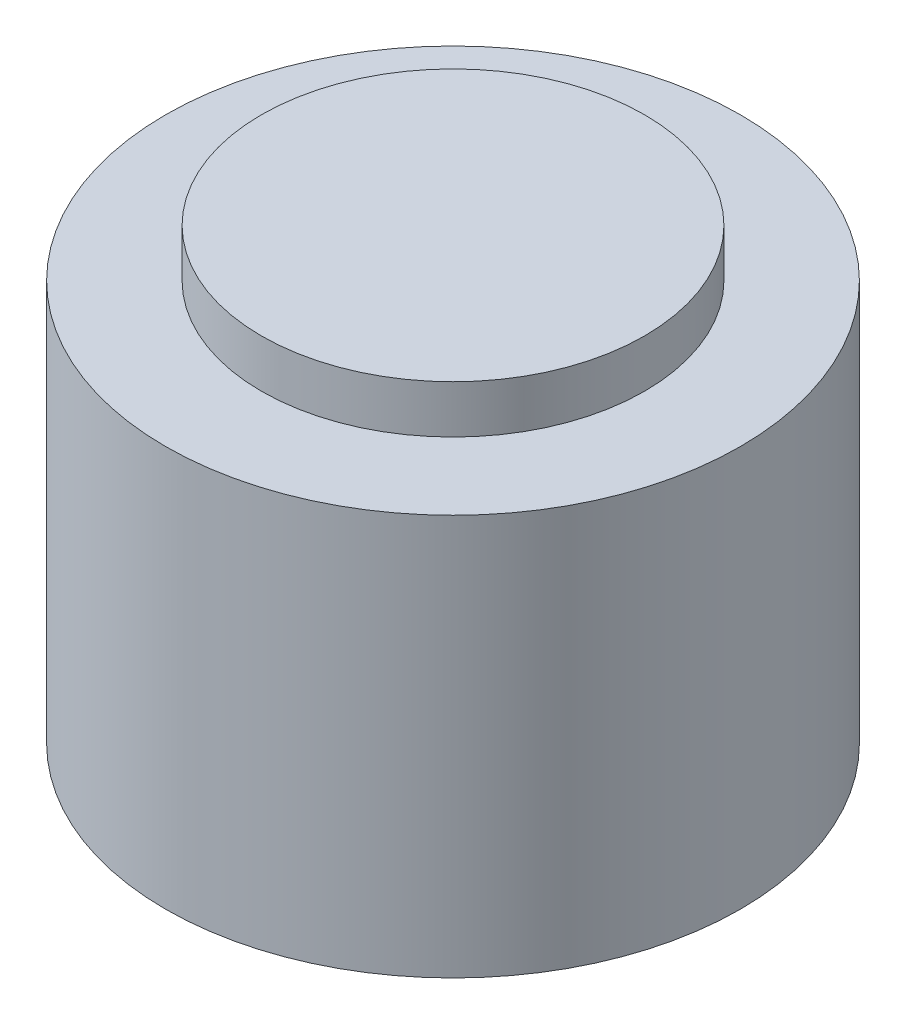
SolidWorks part; units mm, degrees
ref_plane "前视基准面" through (0, 0, 0) normal (0, 0, 1) x (1, 0, 0)
ref_plane "上视基准面" through (0, 0, 0) normal (0, 1, 0) x (1, 0, 0)
ref_plane "右视基准面" through (0, 0, 0) normal (1, 0, 0) x (0, 0, -1)
sketch "草图1" plane through (0, 0, 0) normal (0, 1, 0) x (1, 0, 0)
  circle A0 centre (0, 0) radius 18
  dimension "D1" = 36
extrude "凸台-拉伸1" add sketch "草图1" along normal blind 25.1
sketch "草图2" plane through (0, 25.1, 0) normal (0, 1, 0) x (1, 0, 0)
  circle A0 centre (0, 0) radius 12
  dimension "D1" = 24
extrude "凸台-拉伸2" add sketch "草图2" along normal blind 3
